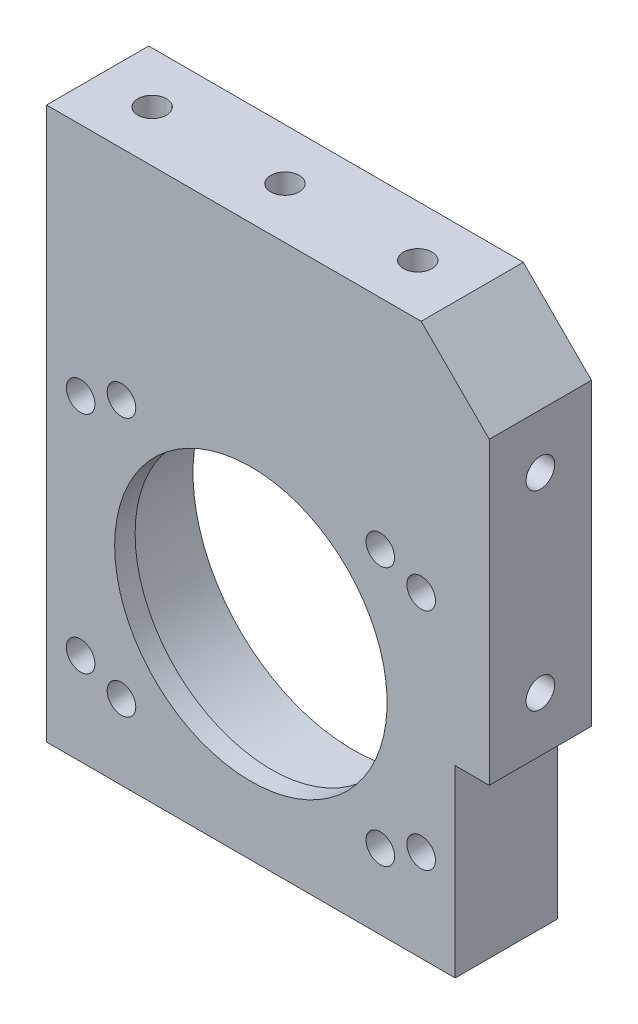
from build123d import *

# Parameters (mm, degrees)
SKETCH_1_W             = 65
SKETCH_1_H             = 82
EXTRUDE_1_DEPTH        = 7.5
SKETCH_10_R            = 23.5
CUT_EXTRUDE_1_DEPTH    = 12
SKETCH_12_R            = 20
CUT_EXTRUDE_2_DEPTH    = 54.677276384
SKETCH_13_W            = 5
SKETCH_13_H            = 27
CUT_EXTRUDE_3_DEPTH    = 55.426556018
HOLE_WIZARD_M5_1_D     = 4.2
HOLE_WIZARD_M5_2_D     = 4.2
MOVE_FACE_1_BY         = 1
HOLE_WIZARD_M5_4_D     = 4.2
HOLE_WIZARD_M5_4_DEPTH = 12.4
HOLE_WIZARD_M5_4_TIP   = 1.2618073
CHAMFER_2_SIZE         = 10
HOLE_WIZARD_M5_3_D     = 4.2
HOLE_WIZARD_M5_3_DEPTH = 12.4
HOLE_WIZARD_M5_3_TIP   = 1.2618073


with BuildPart() as part:
    # 草图1 → 凸台-拉伸1 (new, symmetric)
    with BuildSketch(Plane.XY):
        Rectangle(SKETCH_1_W, SKETCH_1_H)
    extrude(amount=EXTRUDE_1_DEPTH, both=True)

    # 草图10 → 切除-拉伸1 (cut)
    with BuildSketch(Plane.XY.offset(-7.5)):
        with Locations((-2.5, -11)):
            Circle(SKETCH_10_R)
    extrude(amount=CUT_EXTRUDE_1_DEPTH, mode=Mode.SUBTRACT)

    # 草图12 → 切除-拉伸2 (cut, through all)
    with BuildSketch(Plane(origin=(0, 0, 4.5), x_dir=(-1, 0, 0), z_dir=(0, 0, -1))):
        with Locations((2.5, -11)):
            Circle(SKETCH_12_R)
    extrude(amount=-CUT_EXTRUDE_2_DEPTH, mode=Mode.SUBTRACT)

    # 草图13 → 切除-拉伸3 (cut, through all)
    with BuildSketch(Plane.XY.offset(7.5)):
        with Locations((30, -27.5)):
            Rectangle(SKETCH_13_W, SKETCH_13_H)
    extrude(amount=-CUT_EXTRUDE_3_DEPTH, mode=Mode.SUBTRACT)

    # M5 螺纹孔1 (through all)
    with Locations(Plane(origin=(0, 0, -7.5), x_dir=(-1, 0, 0), z_dir=(0, 0, -1))):
        with Locations((-22.5, 5.5), (-22.5, -27.5), (27.5, -27.5), (27.5, 5.5)):
            Hole(HOLE_WIZARD_M5_1_D / 2)

    # M5 螺纹孔2 (through all)
    with Locations(Plane.XY.offset(7.5)):
        with Locations((-21.5, 8), (-21.5, -30), (16.5, -30), (16.5, 8)):
            Hole(HOLE_WIZARD_M5_2_D / 2)

    # Move Face 1: a face moved inward by 1.0
    extrude(part.faces().sort_by_distance((0, 41, 0))[0], amount=MOVE_FACE_1_BY, dir=(0, -1, 0), mode=Mode.SUBTRACT)

    # M5 螺纹孔4
    with Locations(Plane(origin=(32.5, 0, 0), x_dir=(0, 0, -1), z_dir=(1, 0, 0))):
        with Locations((0, -6), (0, 22)):
            Hole(HOLE_WIZARD_M5_4_D / 2, depth=HOLE_WIZARD_M5_4_DEPTH)
            with Locations((0, 0, -(HOLE_WIZARD_M5_4_DEPTH + HOLE_WIZARD_M5_4_TIP / 2))):  # 118° drill point
                Cone(0, HOLE_WIZARD_M5_4_D / 2, HOLE_WIZARD_M5_4_TIP, mode=Mode.SUBTRACT)

    # 倒角2
    chamfer_2_edges = [part.edges().sort_by_distance(p)[0] for p in [
        (32.5, 40, 0),
    ]]
    chamfer(chamfer_2_edges, length=CHAMFER_2_SIZE)

    # M5 螺纹孔3
    with Locations(Plane(origin=(0, 40, 0), x_dir=(1, 0, 0), z_dir=(0, 1, 0))):
        with Locations((-24.5, 0), (-5, 0), (14.5, 0)):
            Hole(HOLE_WIZARD_M5_3_D / 2, depth=HOLE_WIZARD_M5_3_DEPTH)
            with Locations((0, 0, -(HOLE_WIZARD_M5_3_DEPTH + HOLE_WIZARD_M5_3_TIP / 2))):  # 118° drill point
                Cone(0, HOLE_WIZARD_M5_3_D / 2, HOLE_WIZARD_M5_3_TIP, mode=Mode.SUBTRACT)


solid = part.part
